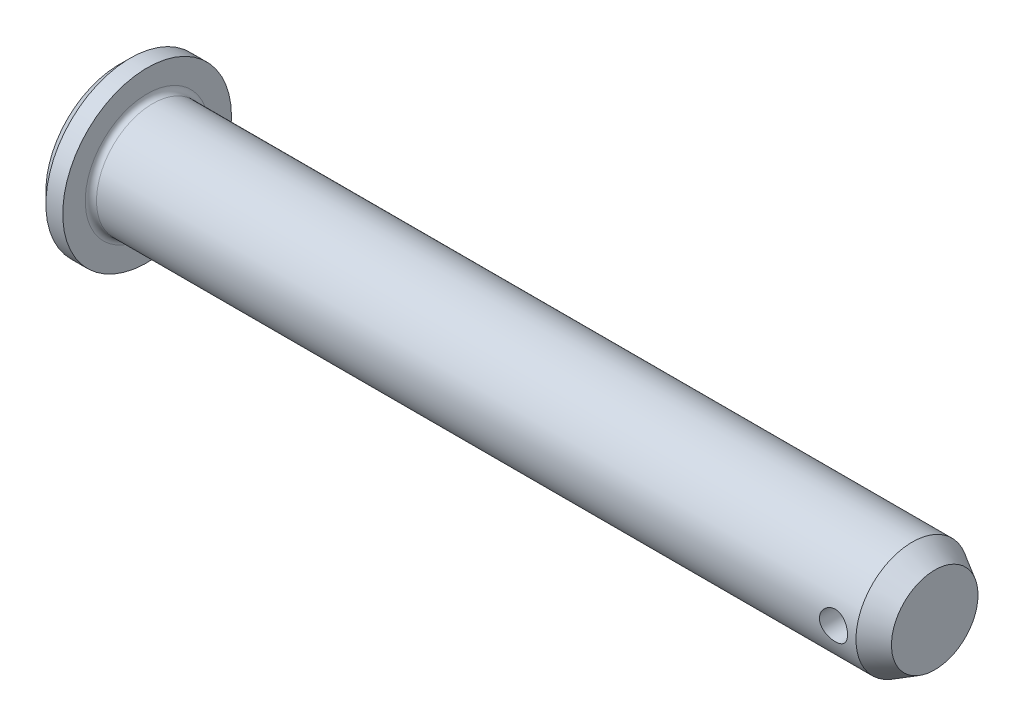
SolidWorks part; units mm, degrees
ref_plane "前视" through (0, 0, 0) normal (0, 0, 1) x (1, 0, 0)
ref_plane "上视" through (0, 0, 0) normal (0, 1, 0) x (1, 0, 0)
ref_plane "右视" through (0, 0, 0) normal (1, 0, 0) x (0, 0, -1)
sketch "尺寸草图" plane through (0, 0, 0) normal (0, 0, 1) x (1, 0, 0)
  line L0 (0, 30) -> (0, 0)
  line L1 (0, 0) -> (140, 0)
  circle A0 centre (132, 0) radius 2.5 construction
  point P3 (0, 20)
  point P5 (5, 0)
  point P6 (1, 0)
  point P7 (136, 0)
  point P8 (7, 0)
  dimension "d1" = 5
  dimension "l" = 140
  dimension "dk" = 30
  dimension "d" = 20
  dimension "k" = 5
  dimension "r" = 1
  dimension "c" = 4
  dimension "e" = 2
  dimension "le" = 8
sketch "草图1" plane through (0, 0, 0) normal (0, 0, 1) x (1, 0, 0)
  line L0 (0, 0) -> (-7.3443, 0) construction
  line L1 (0, 0) -> (145, 0)
  line L2 (0, 0) -> (0, 13)
  line L3 (2, 15) -> (5, 15)
  line L4 (5, 15) -> (5, 10)
  line L5 (5, 10) -> (145, 10)
  line L6 (145, 10) -> (145, 0)
  line L7 (0, 13) -> (2, 15)
  point P4 (0, 15)
  dimension "D2" = 30
  dimension "D1" = 140
  dimension "D3" = 20
  dimension "D4" = 5
revolve "基体-旋转" add sketch "草图1" angle 360 about L0
sketch "草图2" plane through (0, 0, 0) normal (0, 0, 1) x (1, 0, 0)
  line L0 (0, 0) -> (140, 0) construction
  line L1 (145, -10) -> (145, 10) construction
  circle A1 centre (137, 0) radius 2.5
  dimension "D1" = 5
  dimension "D2" = 8
extrude "切除-拉伸1" cut sketch "草图2" against normal through all and the other way through all
fillet "圆角1" radius 1 1 edges at (5, 0, -10)
chamfer "倒角1" distance 4 angle 30 1 edges at (145, 0, -10)
